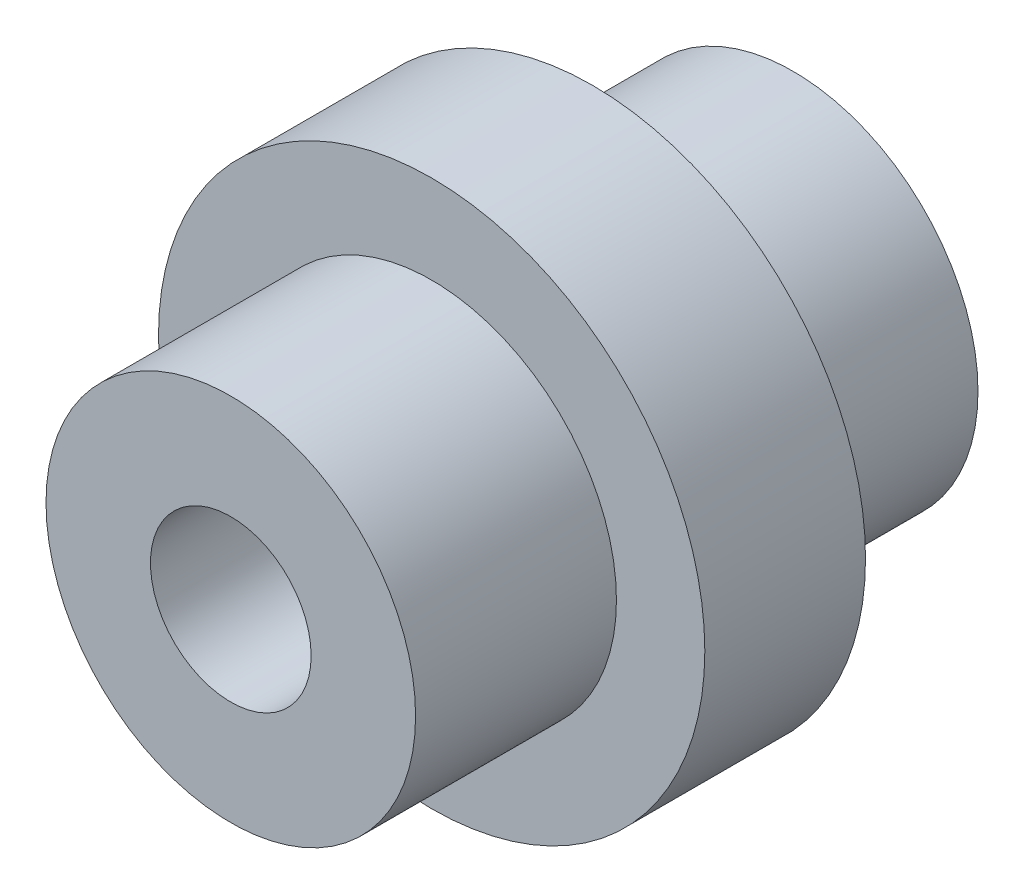
SolidWorks part; units mm, degrees
ref_plane "Front Plane" through (0, 0, 0) normal (0, 0, 1) x (1, 0, 0)
ref_plane "Top Plane" through (0, 0, 0) normal (0, 1, 0) x (1, 0, 0)
ref_plane "Right Plane" through (0, 0, 0) normal (1, 0, 0) x (0, 0, -1)
sketch "Sketch1" plane through (0, 0, 0) normal (0, 0, 1) x (1, 0, 0)
  circle A0 centre (0, 0) radius 34
  dimension "D1" = 68
extrude "Boss-Extrude1" add sketch "Sketch1" along normal mid plane 20
sketch "Sketch2" plane through (0, 0, 10) normal (0, 0, 1) x (1, 0, 0)
  circle A0 centre (0, 0) radius 23
  dimension "D1" = 46
extrude "Boss-Extrude2" add sketch "Sketch2" along normal blind 25
mirror "Mirror1" about plane through (0, 0, 0) normal (0, 0, 1) of "Boss-Extrude2"
sketch "Sketch3" plane through (0, 0, 35) normal (0, 0, 1) x (1, 0, 0)
  circle A0 centre (0, 0) radius 10
  dimension "D1" = 20
extrude "Cut-Extrude1" cut sketch "Sketch3" against normal blind 17
sketch "Sketch4" plane through (0, 0, -35) normal (0, 0, -1) x (-1, 0, 0)
  circle A0 centre (0, 0) radius 16
  dimension "D1" = 32
extrude "Cut-Extrude2" cut sketch "Sketch4" against normal blind 17
